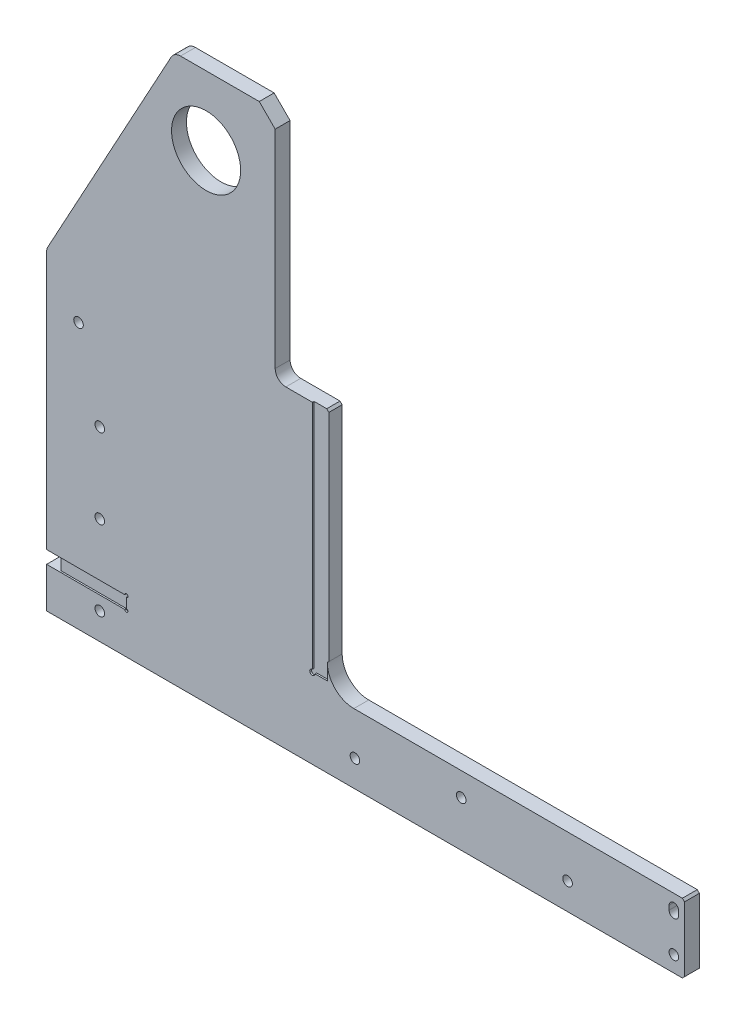
SolidWorks part; units mm, degrees
ref_plane "前视基准面" through (0, 0, 0) normal (0, 0, 1) x (1, 0, 0)
ref_plane "上视基准面" through (0, 0, 0) normal (0, 1, 0) x (1, 0, 0)
ref_plane "右视基准面" through (0, 0, 0) normal (1, 0, 0) x (0, 0, -1)
sketch "草图1" plane through (0, 0, 0) normal (0, 0, 1) x (1, 0, 0)
  line L1 (-300, -257.5) -> (300, -257.5)
  line L2 (-300, -257.5) -> (-300, 257.5)
  line L3 (-300, 257.5) -> (300, 257.5)
  line L4 (300, -257.5) -> (300, 257.5)
  line L5 (-300, -257.5) -> (300, 257.5) construction
  line L6 (-300, 257.5) -> (300, -257.5) construction
  point P0 (0, 0)
  dimension "D1" = 600
  dimension "D2" = 515
extrude "凸台-拉伸1" add sketch "草图1" along normal mid plane 14
sketch "草图2" plane through (0, 0, 7) normal (0, 0, 1) x (1, 0, 0)
  line L0 (300, 257.5) -> (-300, 257.5) construction
  line L1 (-300, 257.5) -> (-300, -257.5) construction
  circle A0 centre (-150, 192.5) radius 32.5
  dimension "D1" = 65
  dimension "D2" = 65
  dimension "D3" = 150
extrude "切除-拉伸1" cut sketch "草图2" against normal up to next
sketch "草图3" plane through (0, 0, -7) normal (0, 0, -1) x (-1, 0, 0)
  line L0 (300, 257.5) -> (300, -257.5) construction
  circle A0 centre (270, -7.5) radius 4.5
  circle A1 centre (250, -82.5) radius 4.5
  circle A2 centre (250, -157.5) radius 4.5
  circle A3 centre (250, -232.5) radius 4.5
  circle A4 centre (150, 192.5) radius 32.5 construction
  circle A5 centre (10, -232.5) radius 4.5
extrude "切除-拉伸2" cut sketch "草图3" against normal up to next
sketch "草图4" plane through (0, 0, -7) normal (0, 0, -1) x (-1, 0, 0)
  line L0 (250, -82.5) -> (250, -157.5) construction
  line L1 (250, -120) -> (56.3441, -120) construction
  line L2 (56, -156) -> (206, -140) construction
  line L3 (56, -100) -> (206, -100)
  line L4 (56, -100) -> (56, -84)
  line L5 (56, -84) -> (206, -84)
  line L6 (206, -100) -> (206, -84)
  line L7 (56, -100) -> (206, -84) construction
  line L8 (56, -84) -> (206, -100) construction
  line L9 (56, -140) -> (206, -156) construction
  line L10 (206, -140) -> (206, -156)
  line L11 (56, -156) -> (206, -156)
  line L12 (56, -140) -> (56, -156)
  line L13 (56, -140) -> (206, -140)
  point P6 (131, -92)
  point P15 (131, -148)
  dimension "D1" = 16
  dimension "D2" = 150
  dimension "D3" = 40
  dimension "D4" = 44
extrude "切除-拉伸3" cut sketch "草图4" against normal blind 1.5
sketch "草图5" plane through (0, 0, -7) normal (0, 0, -1) x (-1, 0, 0)
  circle A0 centre (206, -84) radius 2.5
  circle A1 centre (206, -100) radius 2.5
  circle A2 centre (206, -140) radius 2.5
  circle A3 centre (206, -156) radius 2.5
  circle A4 centre (56, -84) radius 2.5
  circle A5 centre (56, -100) radius 2.5
  circle A6 centre (56, -140) radius 2.5
  circle A7 centre (56, -156) radius 2.5
  dimension "D1" = 5
extrude "切除-拉伸4" cut sketch "草图5" against normal blind 1.5
sketch "草图6" plane through (0, 0, 7) normal (0, 0, 1) x (1, 0, 0)
  line L1 (-300, -219.5) -> (-225, -219.5)
  line L2 (-300, -219.5) -> (-300, -207.5)
  line L3 (-300, -207.5) -> (-225, -207.5)
  line L4 (-225, -219.5) -> (-225, -207.5)
  line L7 (-300, 257.5) -> (-300, -257.5) construction
  circle A1 centre (-250, -232.5) radius 4.5 construction
  point P4 (-300, -213.74)
  dimension "D1" = 13
  dimension "D2" = 12
  dimension "D3" = 75
extrude "切除-拉伸5" cut sketch "草图6" against normal blind 1.5
sketch "草图7" plane through (0, 0, 7) normal (0, 0, 1) x (1, 0, 0)
  circle A0 centre (-225, -207.5) radius 1.5
  circle A1 centre (-225, -219.5) radius 1.5
  dimension "D1" = 3
extrude "切除-拉伸6" cut sketch "草图7" against normal blind 1.5
sketch "草图8" plane through (0, 0, 5.5) normal (0, 0, 1) x (1, 0, 0)
  line L0 (-300, -219.5) -> (-226.5, -219.5) construction
  line L1 (-300, -207.5) -> (-288, -207.5)
  line L2 (-300, -207.5) -> (-300, -219.5)
  line L3 (-300, -219.5) -> (-288, -219.5)
  line L4 (-288, -207.5) -> (-288, -219.5)
  dimension "D1" = 12
extrude "切除-拉伸7" cut sketch "草图8" against normal up to next
sketch "草图9" plane through (0, 0, -7) normal (0, 0, -1) x (-1, 0, 0)
  line L0 (300, -257.5) -> (-300, -257.5) construction
  line L1 (10, -232.5) -> (-190, -232.5) construction
  line L2 (-300, -257.5) -> (-300, 257.5) construction
  line L3 (-290, -204.5) -> (-290, -208.5) construction
  line L4 (-285.5, -204.5) -> (-285.5, -208.5)
  line L5 (-294.5, -204.5) -> (-294.5, -208.5)
  circle A0 centre (-90, -214.5) radius 4.5
  circle A1 centre (-190, -232.5) radius 4.5
  circle A3 centre (-290, -242.5) radius 4.5
  circle A4 centre (10, -232.5) radius 4.5 construction
  arc A5 (-285.5, -204.5) -> (-294.5, -204.5) centre (-290, -204.5) ccw
  arc A6 (-294.5, -208.5) -> (-285.5, -208.5) centre (-290, -208.5) ccw
  point P12 (-290, -206.5)
  dimension "D1" = 9
  dimension "D6" = 9
  dimension "D8" = 4.5
  dimension "D2" = 43
  dimension "D3" = 100
  dimension "D4" = 100
  dimension "D5" = 15
  dimension "D7" = 10
  dimension "D9" = 36
  dimension "D10" = 4
extrude "切除-拉伸8" cut sketch "草图9" against normal up to next
sketch "草图10" plane through (0, 0, -7) normal (0, 0, -1) x (-1, 0, 0)
  line L0 (-300, 257.5) -> (-300, -192.5)
  line L5 (-300, -192.5) -> (36, -192.5)
  line L6 (36, -192.5) -> (36, 37.5)
  line L7 (36, 37.5) -> (85, 37.5)
  line L8 (85, 37.5) -> (85, 257.5)
  line L9 (-300, 257.5) -> (300, 257.5) construction
  line L10 (85, 257.5) -> (-300, 257.5)
  line L12 (56, -86.5) -> (56, -97.5) construction
  line L13 (300, -257.5) -> (-300, -257.5) construction
  dimension "D1" = 385
  dimension "D2" = 230
  dimension "D3" = 20
  dimension "D4" = 65
extrude "切除-拉伸9" cut sketch "草图10" against normal up to next
fillet "圆角1" radius 25 1 edges at (-36, -192.5, 0)
chamfer "倒角1" [suppressed] distance 2 angle 45
sketch "草图11" plane through (0, 0, 7) normal (0, 0, 1) x (1, 0, 0)
  line L1 (-36, 37.5) -> (-50, 37.5)
  line L2 (-36, 37.5) -> (-36, -182.5)
  line L3 (-36, -182.5) -> (-50, -182.5)
  line L4 (-50, 37.5) -> (-50, -182.5)
  dimension "D1" = 220
  dimension "D2" = 14
extrude "切除-拉伸10" cut sketch "草图11" against normal blind 1.5
sketch "草图12" plane through (0, 0, 7) normal (0, 0, 1) x (1, 0, 0)
  circle A0 centre (-50, -182.5) radius 2.5
  dimension "D1" = 5
extrude "切除-拉伸11" cut sketch "草图12" against normal blind 1.5
fillet "圆角2" radius 10 1 edges at (-85, 37.5, 0)
chamfer "倒角2" distance 2 angle 45 1 edges at (-36, 37.5, -0.75)
chamfer "倒角3" distance 2 angle 45 2 edges at (300, -257.5, 0) (300, -192.5, 0)
sketch "草图13" plane through (0, 0, 7) normal (0, 0, 1) x (1, 0, 0)
  line L0 (-180, 257.5) -> (-300, 37.5)
  line L1 (-85, 257.5) -> (-300, 257.5) construction
  line L3 (-300, 37.5) -> (-300, 257.5)
  line L4 (-300, 257.5) -> (-180, 257.5)
  dimension "D1" = 120
  dimension "D2" = 220
extrude "切除-拉伸12" cut sketch "草图13" against normal up to next
chamfer "倒角4" distance 15 angle 45 1 edges at (-85, 257.5, 0)
fillet "圆角3" radius 10 2 edges at (-300, 37.5, 0) (-180, 257.5, 0)
equation "\"D5@草图3\"=\"D4@草图3\""
equation "\"D6@草图3\"=\"D4@草图3\""
